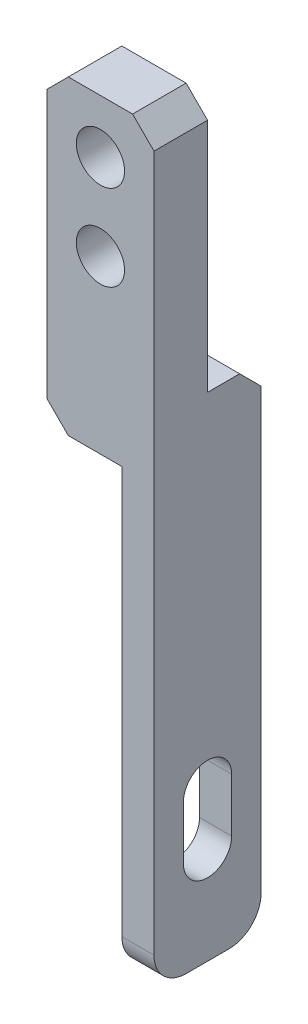
SolidWorks part; units mm, degrees
material "S45C"
ref_plane "Front Plane" through (0, 0, 0) normal (0, 0, 1) x (1, 0, 0)
ref_plane "Top Plane" through (0, 0, 0) normal (0, 1, 0) x (1, 0, 0)
ref_plane "Right Plane" through (0, 0, 0) normal (1, 0, 0) x (0, 0, -1)
sketch "Sketch1" plane through (0, 0, 0) normal (0, 0, 1) x (1, 0, 0)
  line L1 (-5, -35) -> (5, -35)
  line L2 (-5, -35) -> (-5, 35)
  line L3 (-5, 35) -> (5, 35)
  line L4 (5, -35) -> (5, 35)
  line L5 (-5, -35) -> (5, 35) construction
  line L6 (-5, 35) -> (5, -35) construction
  point P0 (0, 0)
  dimension "D1" = 10
  dimension "D2" = 70
extrude "Boss-Extrude1" add sketch "Sketch1" along normal mid plane 10
sketch "Sketch2" plane through (0, 0, 5) normal (0, 0, 1) x (1, 0, 0)
  line L1 (2, -35) -> (-5, -35)
  line L2 (2, -35) -> (2, 6)
  line L3 (2, 6) -> (-5, 6)
  line L4 (-5, -35) -> (-5, 6)
  line L5 (5, -35) -> (5, 35) construction
  dimension "D1" = 41
  dimension "D2" = 3
extrude "Cut-Extrude1" cut sketch "Sketch2" against normal through all
sketch "Sketch3" plane through (5, 0, 0) normal (1, 0, 0) x (0, 0, -1)
  line L0 (-5, -35) -> (-5, 35) construction
  line L1 (5, 35) -> (0, 35)
  line L2 (5, 35) -> (5, 11)
  line L3 (5, 11) -> (0, 11)
  line L4 (0, 35) -> (0, 11)
  dimension "D1" = 5
  dimension "D2" = 24
extrude "Cut-Extrude2" cut sketch "Sketch3" against normal through all
sketch "Sketch4" plane through (-5, 0, 0) normal (-1, 0, 0) x (0, 0, 1)
  line L0 (0, -21) -> (0, -26) construction
  line L1 (2.25, -21) -> (2.25, -26)
  line L2 (-2.25, -21) -> (-2.25, -26)
  line L3 (5, -35) -> (-5, -35) construction
  arc A0 (2.25, -21) -> (-2.25, -21) centre (0, -21) ccw
  arc A1 (-2.25, -26) -> (2.25, -26) centre (0, -26) ccw
  point P3 (0, -23.5)
  dimension "D3" = 2.25
  dimension "D1" = 5
  dimension "D2" = 11.5
extrude "Cut-Extrude3" cut sketch "Sketch4" against normal through all
fillet "Fillet1" radius 3 2 edges at (3.5, -35, -5) (3.5, -35, 5)
hole_wizard "M4 Clearance Hole1" positions "Sketch6" profile "Sketch5" hole size "M4" standard "GB" end condition through all
sketch "Sketch6" plane through (0, 0, 5) normal (0, 0, 1) x (1, 0, 0)
  line L0 (5, 35) -> (-5, 35) construction
  point P0 (0, 30)
  point P2 (0, 22)
  dimension "D1" = 5
  dimension "D2" = 8
sketch "Sketch5" plane through (0, 30, 5) normal (1, 0, 0) x (0, -1, 0)
  line L0 (0, 0) -> (0, 10)
  line L1 (0, 10) -> (2.25, 10)
  line L2 (2.25, 10) -> (2.25, 0)
  line L5 (2.25, 0) -> (0, 0)
  line L11 (0, -6.35) -> (0, 107.95) construction
  dimension "通孔孔直径" = 4.5
  dimension "通孔孔深度" = 10
chamfer "Chamfer1" distance 2 angle 45 4 edges at (0, 11, -5) (-5, 35, 2.5) (5, 35, 2.5) (-5, 6, 0)
